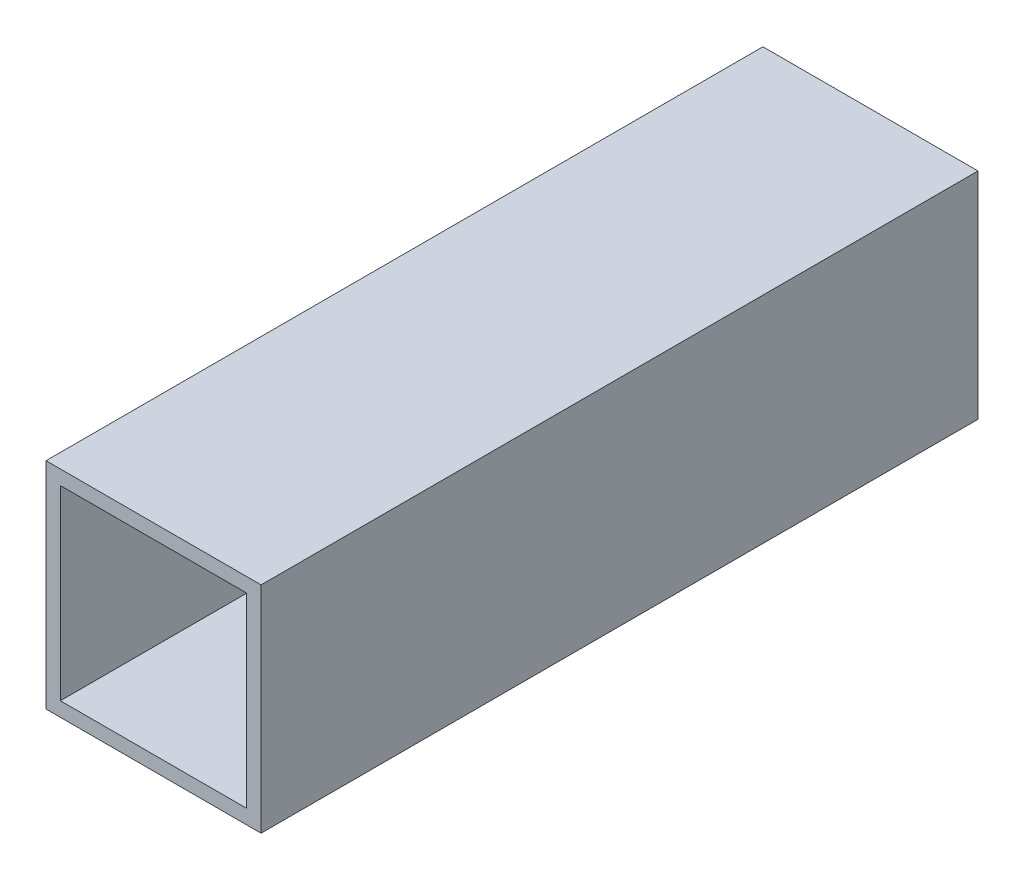
SolidWorks part; units mm, degrees
ref_plane "前视基准面" through (0, 0, 0) normal (0, 0, 1) x (1, 0, 0)
ref_plane "上视基准面" through (0, 0, 0) normal (0, 1, 0) x (1, 0, 0)
ref_plane "右视基准面" through (0, 0, 0) normal (1, 0, 0) x (0, 0, -1)
sketch "草图1" plane through (0, 0, 0) normal (0, 0, 1) x (1, 0, 0)
  line L0 (13, -13) -> (13, 13)
  line L1 (15, -15) -> (-15, -15)
  line L2 (15, -15) -> (15, 15)
  line L3 (15, 15) -> (-15, 15)
  line L4 (-15, -15) -> (-15, 15)
  line L5 (15, -15) -> (-15, 15) construction
  line L6 (15, 15) -> (-15, -15) construction
  line L7 (13, 13) -> (-13, 13)
  line L8 (-13, -13) -> (-13, 13)
  line L9 (13, -13) -> (-13, -13)
  point P0 (0, 0)
  dimension "D1" = 30
  dimension "D2" = 2
extrude "凸台-拉伸1" add sketch "草图1" along normal mid plane 100
